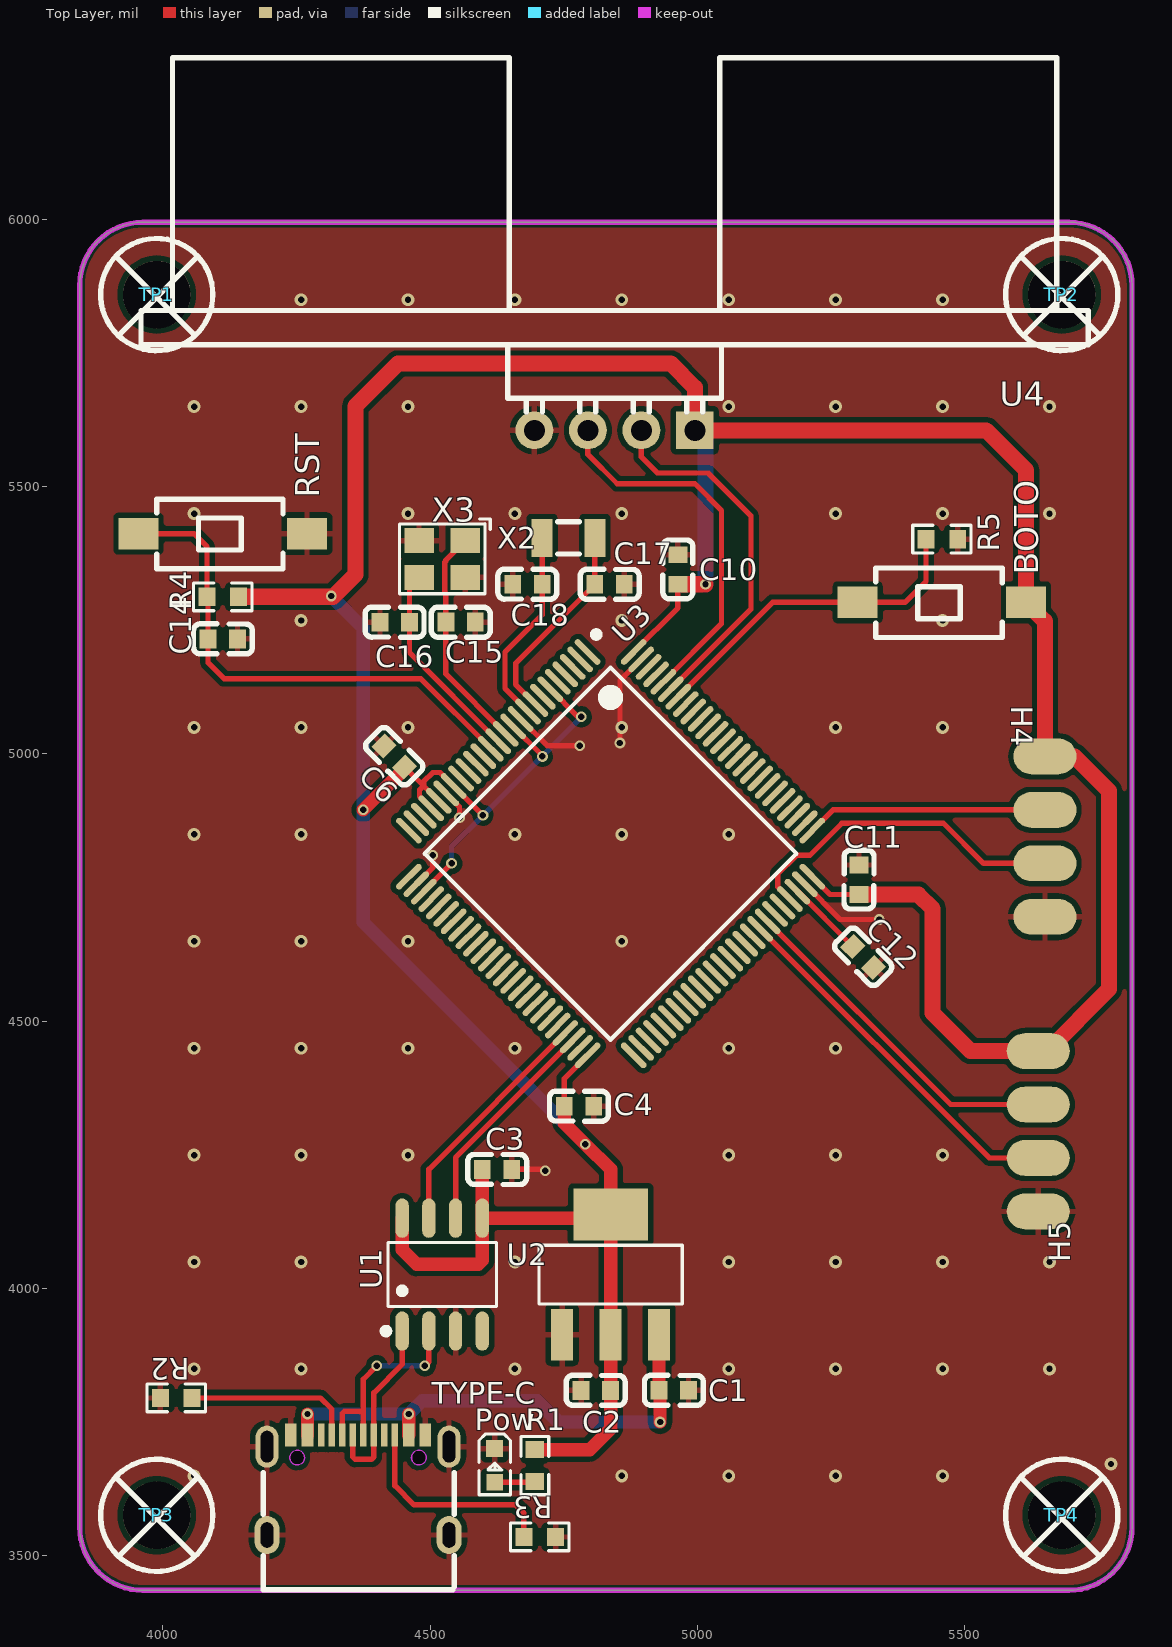
[diagram p0: Top Layer view]
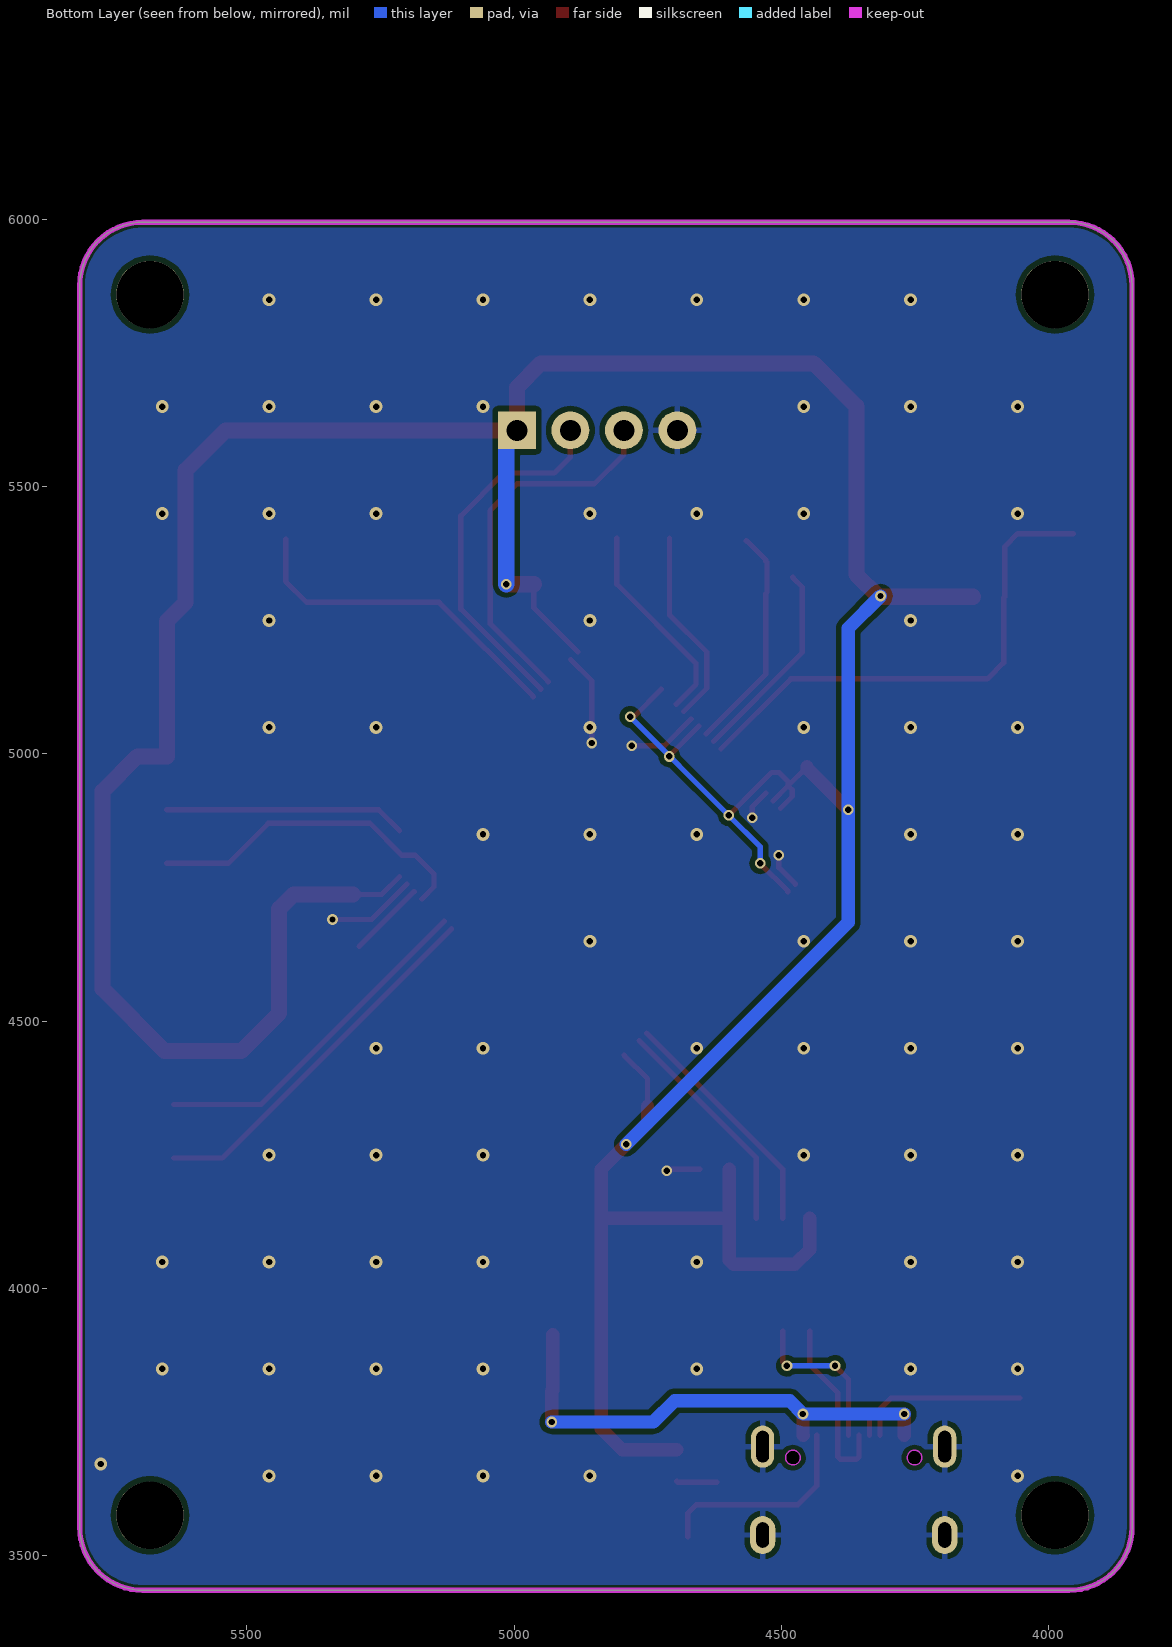
[diagram p1: Bottom Layer view, seen from below]
# Altium PCB MISC61235.pcbdoc
Units mil, origin at the board's own origin, x right, y up, seen from the top; angles counter-clockwise.
Board outline 1968.5 x 2559.06 mil, 2 copper layers (Top Layer, Bottom Layer), stack 62.205 mil thick; 34 components, 93 nets, 192 pads, 90 vias.

## Layer stack, top to bottom
Top Solder Mask Layer: solder mask 0.394, Dk 3.3
Top Layer: signal copper 1.378
Dielectric1: surface 59.449, FR4, Dk 4.5
Bottom Layer: signal copper 1.378
Bottom Solder Mask Layer: solder mask 0.394, Dk 3.3

## Board outline
3962.51,5994.18 ccw(c3962.51,5876.07) 3844.4,5876.07 3844.4,3553.24 ccw(c3962.51,3553.24) 3962.51,3435.13 5694.79,3435.13 ccw(c5694.79,3553.24) 5812.9,3553.24 5812.9,5876.07 ccw(c5694.79,5876.07) 5694.79,5994.18

## Design rules (kind name [scope] priority, off if disabled: settings)
BoardOutlineClearance copperThickness2oz_1 [All] p2 off: genericclearance=7.99 ignorepadtopadclearanceinfootprint=FALSE except(0: Arc-SplitContinuation Track-SplitContinuation SMDPad-SplitContinuation THPad-SplitContinuation Via-SplitContinuation Fill-SplitContinuation Region-SplitContinuation Poly-SplitContinuation Text-SplitContinuation Hole-SplitContinuation; 5.98: SMDPad-CutoutEdge THPad-CutoutEdge Via-CutoutEdge Fill-CutoutEdge Region-CutoutEdge Text-CutoutEdge Hole-CutoutEdge; 10: Poly-OutlineEdge Poly-CutoutEdge; 11.81: Arc-OutlineEdge Track-OutlineEdge SMDPad-OutlineEdge THPad-OutlineEdge Via-OutlineEdge Fill-OutlineEdge Region-OutlineEdge Text-OutlineEdge Hole-OutlineEdge Arc-CutoutEdge Track-CutoutEdge)
BoardOutlineClearance Plane_innerPlane_1 [All] p4 off: genericclearance=4.02 ignorepadtopadclearanceinfootprint=FALSE except(0: Arc-SplitContinuation Track-SplitContinuation SMDPad-SplitContinuation THPad-SplitContinuation Via-SplitContinuation Fill-SplitContinuation Region-SplitContinuation Poly-SplitContinuation Text-SplitContinuation Hole-SplitContinuation; 5.98: SMDPad-CutoutEdge THPad-CutoutEdge Via-CutoutEdge Fill-CutoutEdge Region-CutoutEdge Text-CutoutEdge Hole-CutoutEdge; 10: Poly-OutlineEdge Poly-CutoutEdge; 11.81: Arc-OutlineEdge Track-OutlineEdge SMDPad-OutlineEdge THPad-OutlineEdge Via-OutlineEdge Fill-OutlineEdge Region-OutlineEdge Text-OutlineEdge Hole-OutlineEdge Arc-CutoutEdge Track-CutoutEdge)
BoardOutlineClearance Copper_copperRegion_1 [All] p6 off: genericclearance=4.02 ignorepadtopadclearanceinfootprint=FALSE except(0: Arc-SplitContinuation Track-SplitContinuation SMDPad-SplitContinuation THPad-SplitContinuation Via-SplitContinuation Fill-SplitContinuation Region-SplitContinuation Poly-SplitContinuation Text-SplitContinuation Hole-SplitContinuation; 5.98: SMDPad-CutoutEdge THPad-CutoutEdge Via-CutoutEdge Fill-CutoutEdge Region-CutoutEdge Text-CutoutEdge Hole-CutoutEdge; 10: Poly-OutlineEdge Poly-CutoutEdge; 11.81: Arc-OutlineEdge Track-OutlineEdge SMDPad-OutlineEdge THPad-OutlineEdge Via-OutlineEdge Fill-OutlineEdge Region-OutlineEdge Text-OutlineEdge Hole-OutlineEdge Arc-CutoutEdge Track-CutoutEdge)
BoardOutlineClearance Copper_copperRegion1_1 [All] p8 off: genericclearance=4.02 ignorepadtopadclearanceinfootprint=FALSE except(0: Arc-SplitContinuation Track-SplitContinuation SMDPad-SplitContinuation THPad-SplitContinuation Via-SplitContinuation Fill-SplitContinuation Region-SplitContinuation Poly-SplitContinuation Text-SplitContinuation Hole-SplitContinuation; 5.98: SMDPad-CutoutEdge THPad-CutoutEdge Via-CutoutEdge Fill-CutoutEdge Region-CutoutEdge Text-CutoutEdge Hole-CutoutEdge; 10: Poly-OutlineEdge Poly-CutoutEdge; 11.81: Arc-OutlineEdge Track-OutlineEdge SMDPad-OutlineEdge THPad-OutlineEdge Via-OutlineEdge Fill-OutlineEdge Region-OutlineEdge Text-OutlineEdge Hole-OutlineEdge Arc-CutoutEdge Track-CutoutEdge)
BoardOutlineClearance copperThickness1oz_1 [All] p10: genericclearance=4.02 ignorepadtopadclearanceinfootprint=FALSE except(0: Arc-SplitContinuation Track-SplitContinuation SMDPad-SplitContinuation THPad-SplitContinuation Via-SplitContinuation Fill-SplitContinuation Region-SplitContinuation Poly-SplitContinuation Text-SplitContinuation Hole-SplitContinuation; 5.98: SMDPad-CutoutEdge THPad-CutoutEdge Via-CutoutEdge Fill-CutoutEdge Region-CutoutEdge Text-CutoutEdge Hole-CutoutEdge; 10: Poly-OutlineEdge Poly-CutoutEdge; 11.81: Arc-OutlineEdge Track-OutlineEdge SMDPad-OutlineEdge THPad-OutlineEdge Via-OutlineEdge Fill-OutlineEdge Region-OutlineEdge Text-OutlineEdge Hole-OutlineEdge Arc-CutoutEdge Track-CutoutEdge)
Clearance copperThickness2oz [All] p1 off: gap=7.99 ignorepadtopadclearanceinfootprint=FALSE except(5.98: SMDPad-Track SMDPad-SMDPad THPad-Track SMDPad-THPad THPad-THPad Track-Via SMDPad-Via THPad-Via Via-Via Fill-Track Region-Track Fill-SMDPad Region-SMDPad Fill-THPad Region-THPad Fill-Via Region-Via Fill-Fill Fill-Region Region-Region Arc-Track Arc-SMDPad Arc-THPad Arc-Via Fill-Arc Region-Arc Arc-Arc Text-Track SMDPad-Text Text-THPad Text-Via Fill-Text Region-Text Arc-Text Text-Text Hole-Track Hole-SMDPad Hole-THPad Hole-Via Fill-Hole Region-Hole Hole-Arc Hole-Text; 10: Poly-Track Poly-SMDPad Poly-THPad Poly-Via Poly-Fill Poly-Region Poly-Poly Poly-Arc Poly-Text Poly-Hole)
Clearance Plane_innerPlane [All] p3 off: gap=4.02 ignorepadtopadclearanceinfootprint=FALSE except(5.98: SMDPad-Track SMDPad-SMDPad THPad-Track SMDPad-THPad THPad-THPad Fill-Track Region-Track Fill-SMDPad Region-SMDPad Fill-THPad Region-THPad Fill-Via Region-Via Fill-Fill Fill-Region Region-Region Arc-Track Arc-SMDPad Arc-THPad Arc-Via Fill-Arc Region-Arc Arc-Arc Text-Track SMDPad-Text Text-THPad Text-Via Fill-Text Region-Text Arc-Text Text-Text Hole-Track Hole-SMDPad Hole-THPad Fill-Hole Region-Hole Hole-Arc Hole-Text; 10: Poly-Track Poly-SMDPad Poly-THPad Poly-Via Poly-Fill Poly-Region Poly-Poly Poly-Arc Poly-Text Poly-Hole)
Clearance Copper_copperRegion [All] p5 off: gap=4.02 ignorepadtopadclearanceinfootprint=FALSE except(5.98: SMDPad-Track SMDPad-SMDPad THPad-Track SMDPad-THPad THPad-THPad Fill-Track Region-Track Fill-SMDPad Region-SMDPad Fill-THPad Region-THPad Fill-Via Region-Via Fill-Fill Fill-Region Region-Region Arc-Track Arc-SMDPad Arc-THPad Arc-Via Fill-Arc Region-Arc Arc-Arc Text-Track SMDPad-Text Text-THPad Text-Via Fill-Text Region-Text Arc-Text Text-Text Hole-Track Hole-SMDPad Hole-THPad Fill-Hole Region-Hole Hole-Arc Hole-Text; 10: Poly-Track Poly-SMDPad Poly-THPad Poly-Via Poly-Fill Poly-Region Poly-Poly Poly-Arc Poly-Text Poly-Hole)
Clearance Copper_copperRegion1 [All] p7 off: gap=4.02 ignorepadtopadclearanceinfootprint=FALSE except(5.98: SMDPad-Track SMDPad-SMDPad THPad-Track SMDPad-THPad THPad-THPad Fill-Track Region-Track Fill-SMDPad Region-SMDPad Fill-THPad Region-THPad Fill-Via Region-Via Fill-Fill Fill-Region Region-Region Arc-Track Arc-SMDPad Arc-THPad Arc-Via Fill-Arc Region-Arc Arc-Arc Text-Track SMDPad-Text Text-THPad Text-Via Fill-Text Region-Text Arc-Text Text-Text Hole-Track Hole-SMDPad Hole-THPad Fill-Hole Region-Hole Hole-Arc Hole-Text; 10: Poly-Track Poly-SMDPad Poly-THPad Poly-Via Poly-Fill Poly-Region Poly-Poly Poly-Arc Poly-Text Poly-Hole)
Clearance copperThickness1oz [All] p9: gap=4.02 ignorepadtopadclearanceinfootprint=FALSE except(5.98: SMDPad-Track SMDPad-SMDPad THPad-Track SMDPad-THPad THPad-THPad Fill-Track Region-Track Fill-SMDPad Region-SMDPad Fill-THPad Region-THPad Fill-Via Region-Via Fill-Fill Fill-Region Region-Region Arc-Track Arc-SMDPad Arc-THPad Arc-Via Fill-Arc Region-Arc Arc-Arc Text-Track SMDPad-Text Text-THPad Text-Via Fill-Text Region-Text Arc-Text Text-Text Hole-Track Hole-SMDPad Hole-THPad Fill-Hole Region-Hole Hole-Arc Hole-Text; 10: Poly-Track Poly-SMDPad Poly-THPad Poly-Via Poly-Fill Poly-Region Poly-Poly Poly-Arc Poly-Text Poly-Hole)
DiffPairsRouting differentialPair [All] p1: maxlimit=10 minlimit=6 mostfreqgap=10 toplayer_minwidth=5 toplayer_prefwidth=10 toplayer_maxwidth=100 toplayer_mingap=6 toplayer_prefgap=10 toplayer_maxgap=10 bottomlayer_minwidth=5 bottomlayer_prefwidth=10 bottomlayer_maxwidth=100 bottomlayer_mingap=6 bottomlayer_prefgap=10 bottomlayer_maxgap=10 maxuncoupledlength=393.7
HoleToHoleClearance otherClearance [All] p1: gap=11.8 allowstackedmicrovias=TRUE
Length netLength [All] p1: minlimit=0 maxlimit=0
PasteMaskExpansion pasteMaskExpansion [All] p1: expansion=0
PlaneConnect innerPlane [All] p1: planeconnectstyle=Relief reliefexpansion=20 reliefentries=4 reliefconductorwidth=10 reliefairgap=10
PolygonConnect copperRegion1 [All] p1 off: connectstyle=Direct reliefconductorwidth=10 reliefentries=4 polygonreliefangle="90 Angle" airgapwidth=10 via.connectstyle=Relief via.reliefconductorwidth=10 via.reliefentries=4 via.polygonreliefangle="90 Angle" via.airgapwidth=10
PolygonConnect copperRegion [All] p2: connectstyle=Relief reliefconductorwidth=10 reliefentries=4 polygonreliefangle="90 Angle" airgapwidth=10 via.connectstyle=Relief via.reliefconductorwidth=10 via.reliefentries=4 via.polygonreliefangle="90 Angle" via.airgapwidth=10
RoutingVias viaSize [All] p1: holewidth=12.01 width=24.02 viastyle="Through Hole" minholewidth=11.81 minwidth=15.71 maxholewidth=247.99 maxwidth=393.7
SolderMaskExpansion solderMaskExpansion [IsVia] p1: expansion=-1000 istentingtop=TRUE
SolderMaskExpansion solderMaskExpansion [All] p2: expansion=2.01 istentingtop=FALSE
Width copperThickness2oz_2 [All] p1 off: maxlimit=100 minlimit=8 preferedwidth=10
Width copperThickness1oz_2 [All] p2: maxlimit=100 minlimit=5 preferedwidth=10

## Components (designator, comment, footprint, x,y, rotation, side; value= is the part's Value field where it differs from the comment)
BOTO "TS-1101-C-W" SW-SMD_L6.0-W3.3-LS8.0 5457.22,5283.12 r0 top
C1 "100nF" C0603 4955.61,3809.36 r180 top
C2 "100nF" C0603 4809.94,3809.14 r0 top
C3 "100nF" C0603 4625.1,4222.53 r180 top
C4 "100nF" C0603 4778.44,4340.64 r0 top
C6 "100nF" C0603 4432.84,4995.03 r315 top
C10 "100nF" C0603 4963.25,5344.58 r270 top
C11 "100nF" C0603 5302.07,4764.18 r270 top
C12 "2.2uf" C0603 5310,4620 r315 top
C14 "100nF" C0603 4112.08,5214.88 r180 top
C15 "20pF" C0603 4556.91,5246.15 r180 top
C16 "20pF" C0603 4433.8,5245.94 r0 top
C17 "12.5pF" C0603 4835.53,5317.02 r180 top
C18 "12.5pF" C0603 4681.99,5317.02 r0 top
H4 "" 侧焊1X4排针 5650,4845 r0 top
H5 "" 侧焊1X4排针 5637.5,4293.87 r180 top
Pow "" LED_0603 4620.96,3666.66 r270 top
R1 "1K" R0603 4695.77,3668.54 r270 top
R2 "5.1K" R0603 4025,3795 r0 top
R3 "5.1K" R0603 4705,3535 r180 top
R4 "10K" R0603 4112.08,5293.62 r0 top
R5 "10K" R0603 5457.22,5401.23 r180 top
RST "TS-1101-C-W" SW-SMD_L6.0-W3.3-LS8.0 4112.08,5411.73 r0 top
TP1 "" M3螺丝 3991.04,5856.39 r0 top
TP2 "" M3螺丝 5683.96,5856.39 r0 top
TP3 "" M3螺丝 3991.04,3572.92 r0 top
TP4 "" M3螺丝 5683.96,3572.92 r0 top
TYPE-C "TYPE-C 16PIN 2MD(073)" USB-C-SMD_TYPE-C-6PIN-2MD-073 4365.06,3631.98 r0 top
U1 "CH340N" SOP-8_L4.9-W3.9-P1.27-LS6.0-BL 4522.54,4025.68 r0 top
U2 "LM1117IMPX-3.3/NOPB" SOT-223_L6.5-W3.5-P2.30-LS7.0-BR 4837.5,4025.68 r270 top
U3 "" LQFP-100_L14.0-W14.0-P0.50-LS16.0-BL 4837.5,4813.08 r225 top
U4 "HC-SR04" TH_HC-SR04V 4845,5605 r180 top
X2 "32.768kHz" FC-135R_L3.2-W1.5 4758.76,5403.63 r180 top
X3 "12MHz" OSC-SMD_4P-L3.2-W2.5-BL 4522.54,5364.26 r180 top

## Footprints (in the part's own frame and the unit in brackets; to place one, negate y for a bottom-side part, rotate by r counter-clockwise, add the part's x,y. Pads: shape width x height; smd on the part's side, far side on the other; paste and mask are expansions set on the pad)
C0603 [mm]
  rect 0.8x0.9 smd: 1(-0.7,0) 2(0.7,0)
  silkscreen extent -1.41,-0.71 1.39,0.72
FC-135R_L3.2-W1.5 [mm]
  rect 1x1.8 smd: 1(-1.25,0) 2(1.25,0)
  silkscreen extent -0.51,-0.76 0.51,0.76
LED_0603 [mil]
  rect 31.5x31.5 smd paste+0 mask+2: 1(-33.5,-0.4) 2(29.5,-0.2)
  silkscreen extent -61,-30 53,30
LQFP-100_L14.0-W14.0-P0.50-LS16.0-BL [mm]
  oval 0.3x1.6 smd paste-100 mask+0.051: 1(-6,-7.55) 2(-5.5,-7.55) 3(-5,-7.55) 4(-4.5,-7.55) 5(-4,-7.55) 6(-3.5,-7.55) 7(-3,-7.55) 8(-2.5,-7.55) 9(-2,-7.55) 10(-1.5,-7.55) 11(-1,-7.55) 12(-0.5,-7.55) 13(0,-7.55) 14(0.5,-7.55) 15(1,-7.55) 16(1.5,-7.55) 17(2,-7.55) 18(2.5,-7.55) 19(3,-7.55) 20(3.5,-7.55) 21(4,-7.55) 22(4.5,-7.55) 23(5,-7.55) 24(5.5,-7.55) 25(6,-7.55) 51(6,7.55) 52(5.5,7.55) 53(5,7.55) 54(4.5,7.55) 55(4,7.55) 56(3.5,7.55) 57(3,7.55) 58(2.5,7.55) 59(2,7.55) 60(1.5,7.55) 61(1,7.55) 62(0.5,7.55) 63(0,7.55) 64(-0.5,7.55) 65(-1,7.55) 66(-1.5,7.55) 67(-2,7.55) 68(-2.5,7.55) 69(-3,7.55) 70(-3.5,7.55) 71(-4,7.55) 72(-4.5,7.55) 73(-5,7.55) 74(-5.5,7.55) 75(-6,7.55)
  oval 1.6x0.3 smd paste-100 mask+0.051: 26(7.55,-6) 27(7.55,-5.5) 28(7.55,-5) 29(7.55,-4.5) 30(7.55,-4) 31(7.55,-3.5) 32(7.55,-3) 33(7.55,-2.5) 34(7.55,-2) 35(7.55,-1.5) 36(7.55,-1) 37(7.55,-0.5) 38(7.55,0) 39(7.55,0.5) 40(7.55,1) 41(7.55,1.5) 42(7.55,2) 43(7.55,2.5) 44(7.55,3) 45(7.55,3.5) 46(7.55,4) 47(7.55,4.5) 48(7.55,5) 49(7.55,5.5) 50(7.55,6) 76(-7.55,6) 77(-7.55,5.5) 78(-7.55,5) 79(-7.55,4.5) 80(-7.55,4) 81(-7.55,3.5) 82(-7.55,3) 83(-7.55,2.5) 84(-7.55,2) 85(-7.55,1.5) 86(-7.55,1) 87(-7.55,0.5) 88(-7.55,0) 89(-7.55,-0.5) 90(-7.55,-1) 91(-7.55,-1.5) 92(-7.55,-2) 93(-7.55,-2.5) 94(-7.55,-3) 95(-7.55,-3.5) 96(-7.55,-4) 97(-7.55,-4.5) 98(-7.55,-5) 99(-7.55,-5.5) 100(-7.55,-6)
  silkscreen extent -7.03,-8 6.25,6.25
M3螺丝 [mil]
  round 126 hole 126 paste+0 mask+4: 1(-2.5,2.5)
  silkscreen extent -107,-102 102,107
OSC-SMD_4P-L3.2-W2.5-BL [mm]
  rect 1.4x1.2 smd: 1(-1.1,-0.875) 2(1.1,-0.875) 3(1.1,0.875) 4(-1.1,0.875)
  silkscreen extent -2.29,-1.9 2.03,1.65
R0603 [mil]
  rect 31.75x34.02 smd paste-3937.01 mask+2: 1(-29.66,0) 2(29.66,0)
  silkscreen extent -55,-26 55,26
SOP-8_L4.9-W3.9-P1.27-LS6.0-BL [mm]
  oval 0.63x1.865 smd: 1(-1.905,-2.682) 2(-0.635,-2.682) 3(0.635,-2.682) 4(1.905,-2.682) 5(1.905,2.682) 6(0.635,2.682) 7(-0.635,2.682) 8(-1.905,2.682)
  silkscreen extent -2.82,-2.83 2.58,1.52
SOT-223_L6.5-W3.5-P2.30-LS7.0-BR [mm]
  rect 2.465x1.05 smd: 1(2.858,-2.3) 2(2.857,0) 3(2.857,2.3)
  rect 2.465x3.54 smd: 4(-2.857,0)
  silkscreen extent -1.4,-3.4 1.4,3.4
SW-SMD_L6.0-W3.3-LS8.0 [mm]
  rect 1.9x1.5 smd: 1(-4,0) 2(4,0)
  silkscreen extent -3.14,-1.67 2.86,1.63
TH_HC-SR04V [mm]
  rect 1.8x1.8 hole 1.001: 1(-3.81,0)
  round 1.8 hole 1.001: 2(-1.27,0) 3(1.27,0) 4(3.81,0)
  silkscreen extent -22.5,-17.7 22.5,-0.89
USB-C-SMD_TYPE-C-6PIN-2MD-073 [mm]
  rect 0.55x1.1 smd paste-100 mask+0.05: 1(-3.2,2.375) 2(-2.4,2.375) 11(2.4,2.375) 12(3.2,2.375)
  rect 0.3x1.1 smd paste-100 mask+0.05: 3(-1.75,2.375) 4(-1.25,2.375) 5(-0.75,2.375) 6(-0.25,2.375) 7(0.25,2.375) 8(0.75,2.375) 9(1.25,2.375) 10(1.75,2.375)
  oval 1.2x1.8 hole 0.6 slot 1.2 at 90 deg paste+0 mask+0.05: 13(-4.325,-2.375) 14(4.325,-2.375)
  oval 1.1x2 hole 0.6 slot 1.5 at 90 deg paste+0 mask+0.05: 13(-4.325,1.825) 14(4.325,1.825)
  Board Outline Layer circle w0.003: c-2.89,1.305 r0.35
  Board Outline Layer circle w0.003: c2.89,1.305 r0.35
  Board Outline Layer region: -2.54,1.305 -2.575,1.153 -2.672,1.031 -2.812,0.964 -2.968,0.964 -3.108,1.031 -3.205,1.153 -3.24,1.305 -3.24,1.305 -3.205,1.457 -3.108,1.579 -2.968,1.646 -2.812,1.646 -2.672,1.579 -2.575,1.457 -2.54,1.305
  Board Outline Layer region: -2.54,1.305 -2.549,1.227 -2.575,1.153 -2.616,1.087 -2.672,1.031 -2.738,0.99 -2.812,0.964 -2.89,0.955 -2.968,0.964 -3.042,0.99 -3.108,1.031 -3.164,1.087 -3.205,1.153 -3.231,1.227 -3.24,1.305 -3.231,1.383 -3.205,1.457 -3.164,1.523 -3.108,1.579 -3.042,1.62 -2.968,1.646 -2.89,1.655 -2.812,1.646 -2.738,1.62 -2.672,1.579 -2.616,1.523 -2.575,1.457 -2.549,1.383
  Board Outline Layer region: 3.24,1.305 3.205,1.153 3.108,1.031 2.968,0.964 2.812,0.964 2.672,1.031 2.575,1.153 2.54,1.305 2.54,1.305 2.575,1.457 2.672,1.579 2.812,1.646 2.968,1.646 3.108,1.579 3.205,1.457 3.24,1.305
  Board Outline Layer region: 3.24,1.305 3.231,1.227 3.205,1.153 3.164,1.087 3.108,1.031 3.042,0.99 2.968,0.964 2.89,0.955 2.812,0.964 2.738,0.99 2.672,1.031 2.616,1.087 2.575,1.153 2.549,1.227 2.54,1.305 2.549,1.383 2.575,1.457 2.616,1.523 2.672,1.579 2.738,1.62 2.812,1.646 2.89,1.655 2.968,1.646 3.042,1.62 3.108,1.579 3.164,1.523 3.205,1.457 3.231,1.383
  Multi-Layer board cut-out: -2.54,1.305 -2.575,1.153 -2.672,1.031 -2.812,0.964 -2.968,0.964 -3.108,1.031 -3.205,1.153 -3.24,1.305 -3.24,1.305 -3.205,1.457 -3.108,1.579 -2.968,1.646 -2.812,1.646 -2.672,1.579 -2.575,1.457 -2.54,1.305
  Multi-Layer board cut-out: 3.24,1.305 3.205,1.153 3.108,1.031 2.968,0.964 2.812,0.964 2.672,1.031 2.575,1.153 2.54,1.305 2.54,1.305 2.575,1.457 2.672,1.579 2.812,1.646 2.968,1.646 3.108,1.579 3.205,1.457 3.24,1.305
  silkscreen extent -4.5,-4.97 4.57,0.6
侧焊1X4排针 [mm]
  oval 3x1.7 smd: 1(0,3.81) 2(0,1.27) 3(0,-1.27) 4(0,-3.81)

## Via types
v1: diameter 24.02, hole 12, Top Layer to Bottom Layer, 70 vias
v2: diameter 20, hole 12, Top Layer to Bottom Layer, 19 vias
v3: diameter 24, hole 12, Top Layer to Bottom Layer, 1 vias

## Nets (pads, with @x,y where several pads share a name; then routed paths per layer and width w, separated by ;. In a path a pad name is that pad's centre, name@x,y a point inside that pad or via, vN(x,y) a via of type N, cw(c..) or ccw(c..) an arc to the next point about the centre after c; other vN are vias at no path point)
3.3V: BOTO.2 C2.2 C3.2 C4.1 C6.2 C10.2 C11.2 H4.1 H5.4 R1.1 R4.2 U1.5 U1.8 U2.2 U2.4 U3.6 U3.11 U3.19 U3.21 U3.22 U3.28 U3.50 U3.75 U3.100 U4.1 | length 8188.3
  Top Layer w10: C6.2 4487.74,4940.13 ; U3.28 4488.13,4743.13 v2(4540,4795) ; U3.22 4480,4920.02 4480,4932.39 4487.74,4940.13 ; U3.21 4487.74,4940.13 ; v2(4598.73,4884.82) U3.19 4518.55,4965 4505,4965 4487.74,4947.74 4487.74,4940.13 ; U3.11 4710,4996.26 v2(4710,4995) ; U3.6 4776.48,5068.98 v2(4782.89,5068.98) ; C4.1 4750.88,4392.4 U3.50 ; U3.100 4963.25,5272.89 C10.2 ; U3.75 5248.02,4736.62 C11.2
  Top Layer w25: v2(4375,4895) 4452.32,4972.32 C6.2 ; U1.8 4447.54,4072.46 4475,4045 4590,4045 4597.54,4052.54 U1.5 ; C3.2 U1.5 ; R1.1 4798.2,3698.2 4837.5,3737.5 C2.2 U2.2 U2.4 ; C4.1 4750.88,4309.12 v2(4790.34,4269.66) 4837.5,4222.5 U2.4 ; U1.5 4830.61,4131.29 U2.4
  Top Layer w30: R4.2 4318.62,5293.62 4360,5335 4360,5650 4440,5730 4950,5730 4995,5685 U4.1 5540,5605 5614.7,5530.3 BOTO.2 5650,5247.82 H4.1 5705,4995 5770,4930 5770,4560 5653.87,4443.87 H5.4 5511.13,4443.87 5440,4515 5440,4710 5413.38,4736.62 C11.2 ; C10.2 v2(5015,5317.02)
  Bottom Layer w10: v2(4540,4795) 4540,4826.08 v2(4598.73,4884.82) v2(4782.89,5068.98)
  Bottom Layer w25: v2(4315,5295) 4375,5235 v2(4375,4895) 4375,4685 v2(4790.34,4269.66)
  Bottom Layer w30: U4.1 5015,5585 v2(5015,5317.02)
5V: C1.2 TYPE-C.2 TYPE-C.11 U2.3 | length 929.6
  Top Layer w25: TYPE-C.2 v2(4270.57,3765) ; TYPE-C.11 4460,3725.93 v2(4460,3765) ; U2.3@4928.05,3913.18 C1.2 4930,3807.41 v2(4930,3750)
  Bottom Layer w25: v2(4270.57,3765) v2(4460,3765) 4485,3790 4700,3790 4740,3750 v2(4930,3750)
$1N10043: R2.2 TYPE-C.4 | length 318.5
  Top Layer w10: R2.2 4295,3795 4315.85,3774.15 TYPE-C.4
$1N10069: R3.2 TYPE-C.10 | length 401.8
  Top Layer w10: TYPE-C.10 4433.96,3631.04 4470,3595 4660,3595 4675.34,3579.66 R3.2
$1N19278: C12.1 U3.73 | length 146.1
  Top Layer w10: U3.73 5187.91,4742.09 C12.1
$1N24206: Pow.2 R1.2 | length 75.7
  Top Layer w10: Pow.2 4694.05,3637.16 R1.2
BOOT0: BOTO.1 R5.2 U3.94 | length 631.4
  Top Layer w10: U3.94 5140.51,5283.12 BOTO.1 5388.12,5283.12 5427.56,5322.56 R5.2
D+: TYPE-C.6 TYPE-C.8 U1.1 | length 341.4
  Top Layer w10: TYPE-C.6 4355.21,3684.79 4360,3680 4390,3680 4394.58,3684.58 TYPE-C.8 4394.58,3804.58 4447.54,3857.54 U1.1
D-: TYPE-C.5 TYPE-C.7 U1.2 | length 381.4
  Top Layer w10: TYPE-C.5 4335.53,3765.53 4340,3770 4370,3770 4374.9,3765.1 ; TYPE-C.7 4374.9,3765.1 ; v2(4400,3855) 4374.9,3829.9 4374.9,3765.1 ; v2(4490,3855) 4497.54,3862.54 U1.2
  Bottom Layer w10: v2(4400,3855) v2(4490,3855)
GND: C1.1 C2.1 C3.1 C4.2 C6.1 C10.1 C11.1 C12.2 C14.1 C15.1 C16.1 C17.1 C18.1 H4.4 H5.1 Pow.1 R2.1 R3.1 R5.1 RST.2 TYPE-C.1 TYPE-C.12 TYPE-C.13 TYPE-C.14 U1.3 U2.1 U3.10 U3.20 U3.27 U3.74 U3.99 U4.4 X3.2 X3.4 | length 657.3
  Top Layer w10: U3.27 4505,4786.81 v2(4505,4810) ; U3.20 4555,4900.7 v2(4555,4880) ; C3.1 4712.47,4222.53 v2(4715,4220) ; U3.10 4719.1,5015 v2(4780,5015) ; v2(4855,5020) 4855,5136.81 U3.99 ; U3.74 5266.81,4690 v2(5340,4690)
  other v1: 4058.5,3649.23 4858.5,3649.23 5058.5,3649.23 5258.5,3649.23 5458.5,3649.23 4058.5,3849.23 4258.5,3849.23 4658.5,3849.23 5058.5,3849.23 5258.5,3849.23 5458.5,3849.23 5658.5,3849.23 4058.5,4049.23 4258.5,4049.23 4658.5,4049.23 5058.5,4049.23 5258.5,4049.23 5458.5,4049.23 5658.5,4049.23 4058.5,4249.23 4258.5,4249.23 4458.5,4249.23 5058.5,4249.23 5258.5,4249.23 5458.5,4249.23 4058.5,4449.23 4258.5,4449.23 4458.5,4449.23 4658.5,4449.23 5058.5,4449.23 5258.5,4449.23 4058.5,4649.23 4258.5,4649.23 4458.5,4649.23 4858.5,4649.23 4058.5,4849.23 4258.5,4849.23 4658.5,4849.23 4858.5,4849.23 5058.5,4849.23 4058.5,5049.23 4258.5,5049.23 4458.5,5049.23 4858.5,5049.23 5258.5,5049.23 5458.5,5049.23 4258.5,5249.23 4858.5,5249.23 5458.5,5249.23 4058.5,5449.23 4458.5,5449.23 4658.5,5449.23 4858.5,5449.23 5258.5,5449.23 5458.5,5449.23 5658.5,5449.23 4058.5,5649.23 4258.5,5649.23 4458.5,5649.23 5058.5,5649.23 5258.5,5649.23 5458.5,5649.23 5658.5,5649.23 4258.5,5849.23 4458.5,5849.23 4658.5,5849.23 4858.5,5849.23 5058.5,5849.23 5258.5,5849.23 5458.5,5849.23
  other v3: 5773.53,3671.35
NRST: C14.2 R4.1 RST.1 U3.14 | length 951.4
  Top Layer w10: RST.1 4058.27,5411.73 4082.42,5387.58 R4.1 4084.52,5291.52 C14.2 4084.52,5170.48 4115,5140 4482.73,5140 U3.14
OSC32_IN: C17.2 U3.8 X2.1 | length 387.4
  Top Layer w10: U3.8 4660,5129.78 4660,5169.04 C17.2 X2.1
OSC32_OUT: C18.2 U3.9 X2.2 | length 371.3
  Top Layer w10: U3.9 4640,5121.94 4640,5190 4709.55,5259.55 C18.2 X2.2
OSC_IN: C15.2 U3.12 X3.1 | length 424.7
  Top Layer w10: X3.1 4529.35,5362.21 4529.35,5360.03 4527.31,5357.98 4527.31,5301.64 4529.35,5299.6 C15.2 4529.35,5149.06 U3.12
OSC_OUT: C16.2 U3.13 X3.3 | length 382.7
  Top Layer w10: X3.3 4461.36,5311.94 C16.2 4461.36,5189.22 U3.13
PA0: U3.23
PA1: U3.24
PA2: U3.25
PA3: U3.26
PA4: U3.29
PA5: U3.30
PA6: U3.31
PA7: U3.32
PA8: U3.67
PA9: H5.2 U3.68 | length 697.8
  Top Layer w10: U3.68 5545.91,4243.87 H5.2
PA10: H5.3 U3.69 | length 648.2
  Top Layer w10: U3.69 5473.75,4343.87 H5.3
PA11: U3.70
PA12: U3.71
PA13: H4.3 U3.72 | length 626.7
  Top Layer w10: U3.72 5150,4751.14 5150,4775 5185,4810 5210,4810 5270,4870 5460,4870 5535,4795 H4.3
PA14: H4.2 U3.76 | length 451.3
  Top Layer w10: U3.76 5253.49,4895 H4.2
PA15: U3.77
PB0: U3.35
PB1: U3.36
PB2: U3.37
PB3: U3.89
PB4: U3.90
PB5: U3.91
PB6: U3.92
PB7: U3.93
PB8: U3.95 U4.2 | length 686.9
  Top Layer w10: U4.2 4895,5555 4925,5525 5020,5525 5100,5445 5100,5270.46 U3.95
PB9: U3.96 U4.3 | length 703.9
  Top Layer w10: U4.3 4795,5560 4850,5505 4995,5505 5045,5455 5045,5243.29 U3.96
PB10: U1.7 U3.47 | length 452
  Top Layer w10: U1.7 4497.54,4222.56 U3.47
PB11: U1.6 U3.48 | length 423.1
  Top Layer w10: U1.6 4547.54,4244.73 U3.48
PB12: U3.51
PB13: U3.52
PB14: U3.53
PB15: U3.54
PC0: U3.15
PC1: U3.16
PC2: U3.17
PC3: U3.18
PC4: U3.33
PC5: U3.34
PC6: U3.63
PC7: U3.64
PC8: U3.65
PC9: U3.66
PC10: U3.78
PC11: U3.79
PC12: U3.80
PC13: U3.7
PD0: U3.81
PD1: U3.82
PD2: U3.83
PD3: U3.84
PD4: U3.85
PD5: U3.86
PD6: U3.87
PD7: U3.88
PD8: U3.55
PD9: U3.56
PD10: U3.57
PD11: U3.58
PD12: U3.59
PD13: U3.60
PD14: U3.61
PD15: U3.62
PE0: U3.97
PE1: U3.98
PE2: U3.1
PE3: U3.2
PE4: U3.3
PE5: U3.4
PE6: U3.5
PE7: U3.38
PE8: U3.39
PE9: U3.40
PE10: U3.41
PE11: U3.42
PE12: U3.43
PE13: U3.44
PE14: U3.45
PE15: U3.46
pads on no net: TP1.1 TP2.1 TP3.1 TP4.1 TYPE-C.3 TYPE-C.9 U1.4 U3.49

## Polygon pours and split planes (outlines as drawn)
GND on Top Layer (solid, remove dead copper, pour order 0): 3000,6350 3000,3000 6760,3000 6760,6350
GND on Bottom Layer (solid, remove dead copper, pour order 2): 3575,6280 3575,3035 6105,3035 6105,6280

## Keep-outs
Board Outline Layer:
  the board outline again, w10